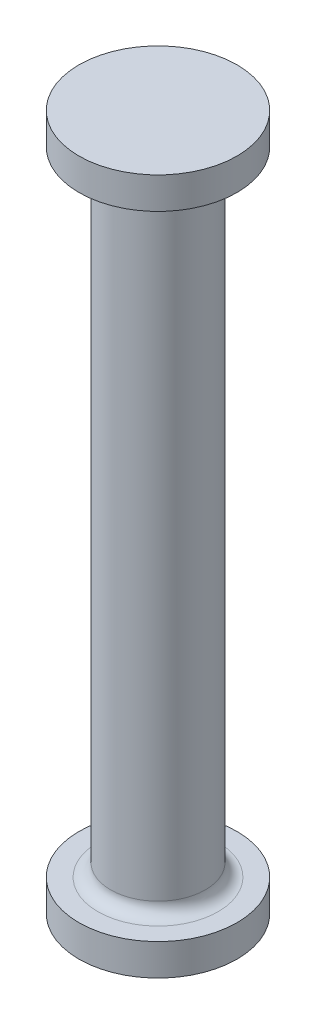
SolidWorks part; units mm, degrees
material "1060 合金"
ref_plane "前视基准面" through (0, 0, 0) normal (0, 0, 1) x (1, 0, 0)
ref_plane "上视基准面" through (0, 0, 0) normal (0, 1, 0) x (1, 0, 0)
ref_plane "右视基准面" through (0, 0, 0) normal (1, 0, 0) x (0, 0, -1)
sketch "草图1" plane through (0, 0, 0) normal (0, 0, 1) x (1, 0, 0)
  line L0 (0, -50) -> (0, 60)
  line L1 (0, 60) -> (12.5, 60)
  line L2 (12.5, 60) -> (12.5, 55)
  line L3 (12.5, 55) -> (7.5, 55)
  line L4 (7.5, 55) -> (7.5, -45)
  line L6 (0, -50) -> (0, 60) construction
  line L7 (12.5, -45) -> (7.5, -45)
  line L8 (12.5, -50) -> (12.5, -45)
  line L9 (0, -50) -> (12.5, -50)
  line L10 (0, 5) -> (24.7444, 5) construction
  dimension "D1" = 12.5
  dimension "D2" = 5
  dimension "D3" = 7.5
  dimension "D4" = 100
  dimension "D5" = 5
revolve "旋转2" add sketch "草图1" angle 360 about L6
fillet "圆角1" radius 2 2 edges at (0, -45, -7.5) (0, 55, -7.5)
